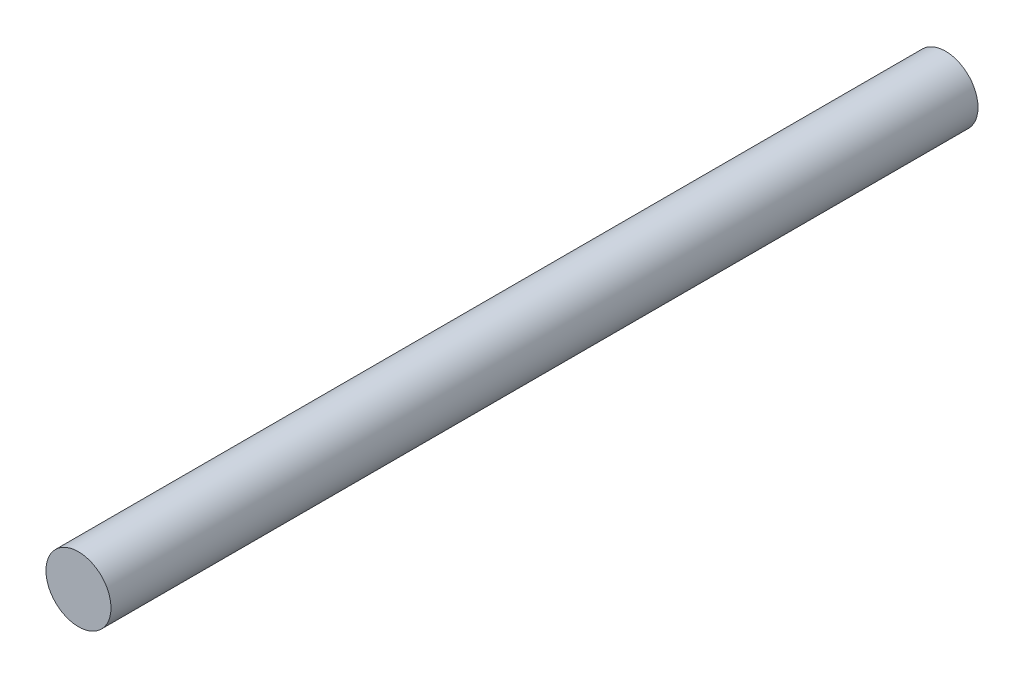
from build123d import *

# Parameters (mm, degrees)
SKETCH_1_R      = 3
EXTRUDE_1_DEPTH = 80


with BuildPart() as part:
    # 草图1 → 凸台-拉伸1 (new body)
    with BuildSketch(Plane.XY):
        Circle(SKETCH_1_R)
    extrude(amount=EXTRUDE_1_DEPTH)


solid = part.part
